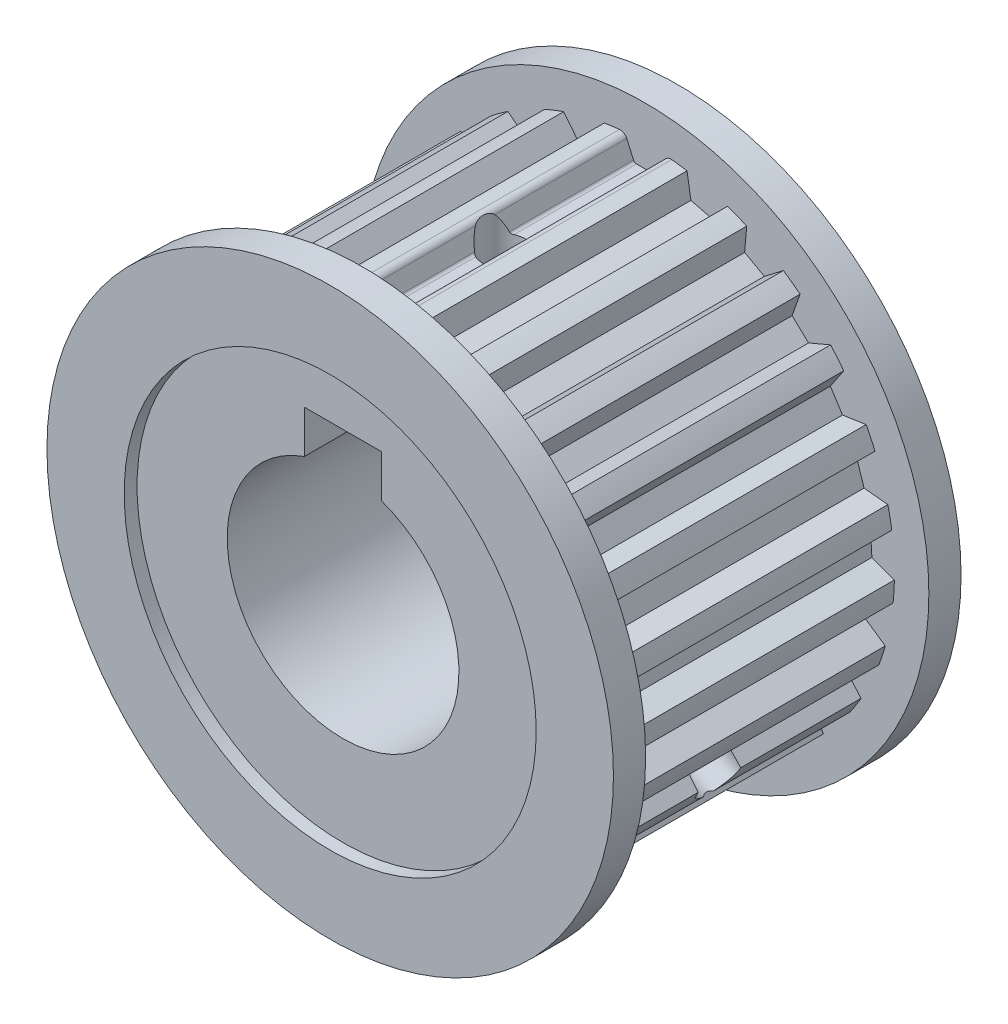
SolidWorks part; units mm, degrees
ref_plane "前视基准面" through (0, 0, 0) normal (0, 0, 1) x (1, 0, 0)
ref_plane "上视基准面" through (0, 0, 0) normal (0, 1, 0) x (1, 0, 0)
ref_plane "右视基准面" through (0, 0, 0) normal (1, 0, 0) x (0, 0, -1)
sketch "草图1" plane through (0, 0, 0) normal (0, 0, 1) x (1, 0, 0)
  circle A0 centre (0, 0) radius 19.325
  dimension "D1" = 38.65
extrude "凸台-拉伸1" add sketch "草图1" along normal mid plane 27
sketch "草图2" plane through (0, 0, 0) normal (0, 0, 1) x (1, 0, 0)
  line L0 (-0.875, 17.555) -> (0.875, 17.555)
  line L1 (-0.875, 17.555) -> (-1.625, 19.2566)
  line L2 (0.875, 17.555) -> (1.625, 19.2566)
  arc A0 (1.625, 19.2566) -> (-1.625, 19.2566) centre (0, 0) ccw
  circle A2 centre (0, 0) radius 19.325 construction
  dimension "D1" = 0.875
  dimension "D2" = 0.875
  dimension "D3" = 1.75
  dimension "D4" = 3.25
  dimension "D5" = 1.625
  dimension "D6" = 17.555
extrude "切除-拉伸1" cut sketch "草图2" against normal mid plane 27
fillet "圆角3" radius 0.55 2 edges at (1.625, 19.2566, 0) (-1.625, 19.2566, 0)
fillet "圆角4" radius 0.25 2 edges at (-0.875, 17.555, 0) (0.875, 17.555, 0)
pattern_circular "阵列(圆周)2" count 25 over 360 about axis through (0, 0, 0) along (0, 0, 1) of "切除-拉伸1"
sketch "草图3" plane through (0, 0, 13.5) normal (0, 0, 1) x (1, 0, 0)
  circle A0 centre (0, 0) radius 22
  dimension "D1" = 44
extrude "凸台-拉伸2" add sketch "草图3" against normal blind 2.5
mirror "镜向1" about plane through (0, 0, 0) normal (0, 0, 1) of "凸台-拉伸2"
sketch "草图4" plane through (0, 0, 13.5) normal (0, 0, 1) x (1, 0, 0)
  circle A0 centre (0, 0) radius 16
  dimension "D1" = 32
extrude "切除-拉伸2" cut sketch "草图4" against normal blind 1
mirror "镜向2" about plane through (0, 0, 0) normal (0, 0, 1) of "切除-拉伸2"
sketch "草图5" plane through (0, 0, 0) normal (0, 0, 1) x (1, 0, 0)
  line L1 (-3, 11.8) -> (3, 11.8)
  line L2 (-3, 11.8) -> (-3, 8.4853)
  line L4 (3, 11.8) -> (3, 8.4853)
  arc A0 (-3, 8.4853) -> (3, 8.4853) centre (0, 0) ccw
  dimension "D1" = 18
  dimension "D4" = 11.8
  dimension "D2" = 6
  dimension "D3" = 3
extrude "切除-拉伸3" cut sketch "草图5" against normal mid plane 27 contours L2 A0 L4 L1
hole_wizard "M4 螺纹孔1" positions "草图7" profile "草图6" tap size "M4" standard "ISO"
sketch "草图7" plane through (0, 0, 0) normal (0, -1, 0) x (-1, 0, 0)
  point P0 (0, 0)
sketch "草图6" plane through (0, 0, 0) normal (1, 0, 0) x (0, 0, -1)
  line L0 (0, 0) -> (0, 30.0526)
  line L1 (0, 30.0526) -> (1.65, 30.0526)
  line L2 (1.65, 30.0526) -> (1.65, 0)
  line L5 (1.65, 0) -> (0, 0)
  line L11 (0, -6.35) -> (0, 107.95) construction
  dimension "通孔螺纹孔钻头直径" = 3.3
  dimension "通孔螺纹孔钻头深度" = 30.0526
cosmetic thread "孔螺蚊线1" parameters "D2"=4
pattern_circular "阵列(圆周)3" count 2 over 120 about axis through (0, 0, 13.5) along (0, 0, -1) of "M4 螺纹孔1"
